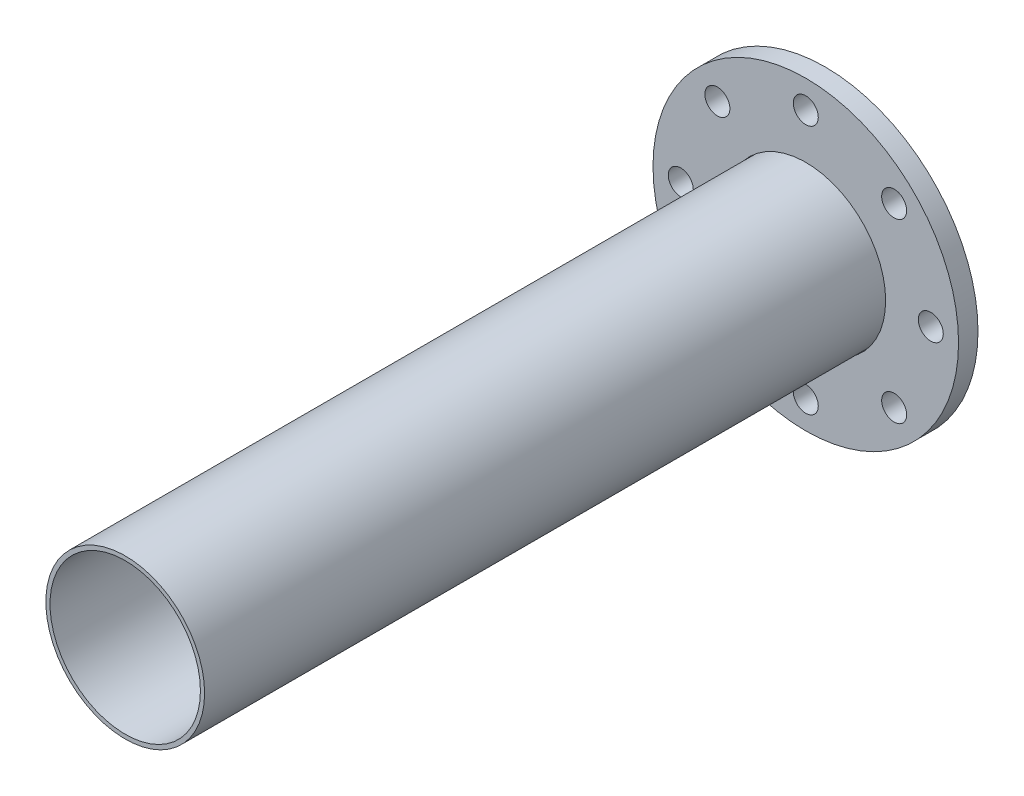
from build123d import *

# Parameters (mm, degrees)
SKETCH1_R           = 110
SKETCH1_R_2         = 57.5
SKETCH1_R_3         = 9
BOSS_EXTRUDE1_DEPTH = 14
SKETCH2_R           = 57.15
SKETCH2_R_2         = 54.15
BOSS_EXTRUDE2_DEPTH = 500


with BuildPart() as part:
    # Sketch1 → Boss-Extrude1 (new body)
    with BuildSketch(Plane.XY):
        Circle(SKETCH1_R)
        Circle(SKETCH1_R_2, mode=Mode.SUBTRACT)
        with Locations((0, 90)):
            Circle(SKETCH1_R_3, mode=Mode.SUBTRACT)
        with Locations((63.639610307, 63.639610307)):
            Circle(SKETCH1_R_3, mode=Mode.SUBTRACT)
        with Locations((90, 0)):
            Circle(SKETCH1_R_3, mode=Mode.SUBTRACT)
        with Locations((63.639610307, -63.639610307)):
            Circle(SKETCH1_R_3, mode=Mode.SUBTRACT)
        with Locations((0, -90)):
            Circle(SKETCH1_R_3, mode=Mode.SUBTRACT)
        with Locations((-63.639610307, -63.639610307)):
            Circle(SKETCH1_R_3, mode=Mode.SUBTRACT)
        with Locations((-90, 0)):
            Circle(SKETCH1_R_3, mode=Mode.SUBTRACT)
        with Locations((-63.639610307, 63.639610307)):
            Circle(SKETCH1_R_3, mode=Mode.SUBTRACT)
    extrude(amount=BOSS_EXTRUDE1_DEPTH)


with BuildPart() as body_2:
    # Sketch2 → Boss-Extrude2 (new body)
    with BuildSketch(Plane.XY.offset(4)):
        Circle(SKETCH2_R)
        Circle(SKETCH2_R_2, mode=Mode.SUBTRACT)
    extrude(amount=BOSS_EXTRUDE2_DEPTH)


solid = Compound([part.part, body_2.part])
